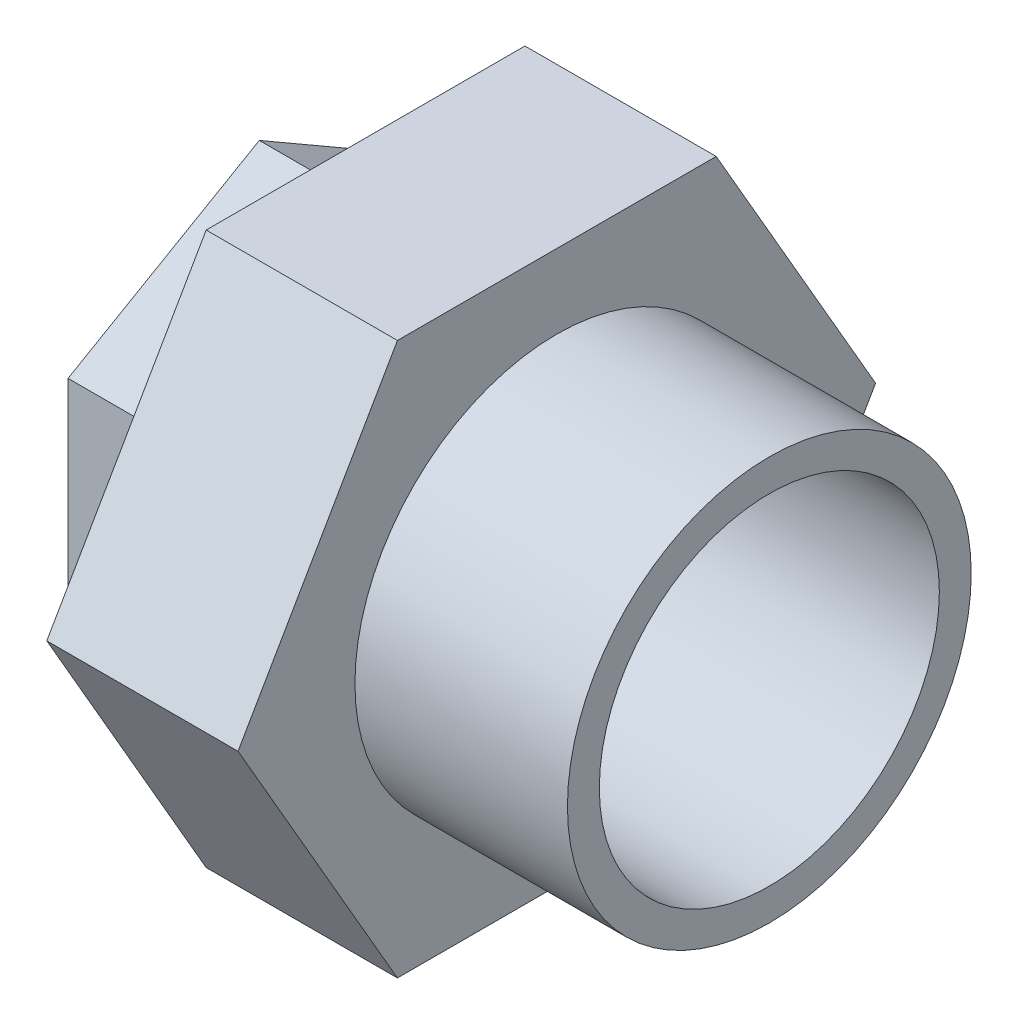
from build123d import *
from build123d.topology import SkipClean

# Parameters (mm, degrees)
SKETCH_1_R        = 19
SKETCH_1_R_2      = 16
EXTRUDE_1_DEPTH   = 20
EXTRUDE_START     = 18
SKETCH_2_R        = 16
EXTRUDE_1_2_DEPTH = 18
SKETCH_3_R        = 16.75
EXTRUDE_2_DEPTH   = 10


with BuildPart() as part:
    # 草图1 → Extrude 1 (new body)
    with BuildSketch(Plane(origin=(0, 0, 0), x_dir=(0, 0, -1), z_dir=(1, 0, 0))):
        Circle(SKETCH_1_R)
        Circle(SKETCH_1_R_2, mode=Mode.SUBTRACT)
    extrude(amount=EXTRUDE_1_DEPTH)

    # 草图2 → Extrude 1 2 (add)
    with SkipClean():  # the faces are left unmerged after this step: merging them gives an invalid solid
        with BuildSketch(Plane.ZY.offset(EXTRUDE_START)):
            Polygon((30, 0), (15, 25.980762114), (-15, 25.980762114), (-30, 0), (-15, -25.980762114), (15, -25.980762114), align=None)
            Circle(SKETCH_2_R, mode=Mode.SUBTRACT)
        extrude(amount=-EXTRUDE_1_2_DEPTH)

    # 草图3 → 凸台-拉伸2 (add)
    with SkipClean():  # the faces are left unmerged after this step: merging them gives an invalid solid
        with BuildSketch(Plane.ZY.offset(18)):
            Polygon((0, 20.784609691), (-18, 10.392304845), (-18, -10.392304845), (0, -20.784609691), (18, -10.392304845), (18, 10.392304845), align=None)
            Circle(SKETCH_3_R, mode=Mode.SUBTRACT)
        extrude(amount=EXTRUDE_2_DEPTH)


solid = part.part
